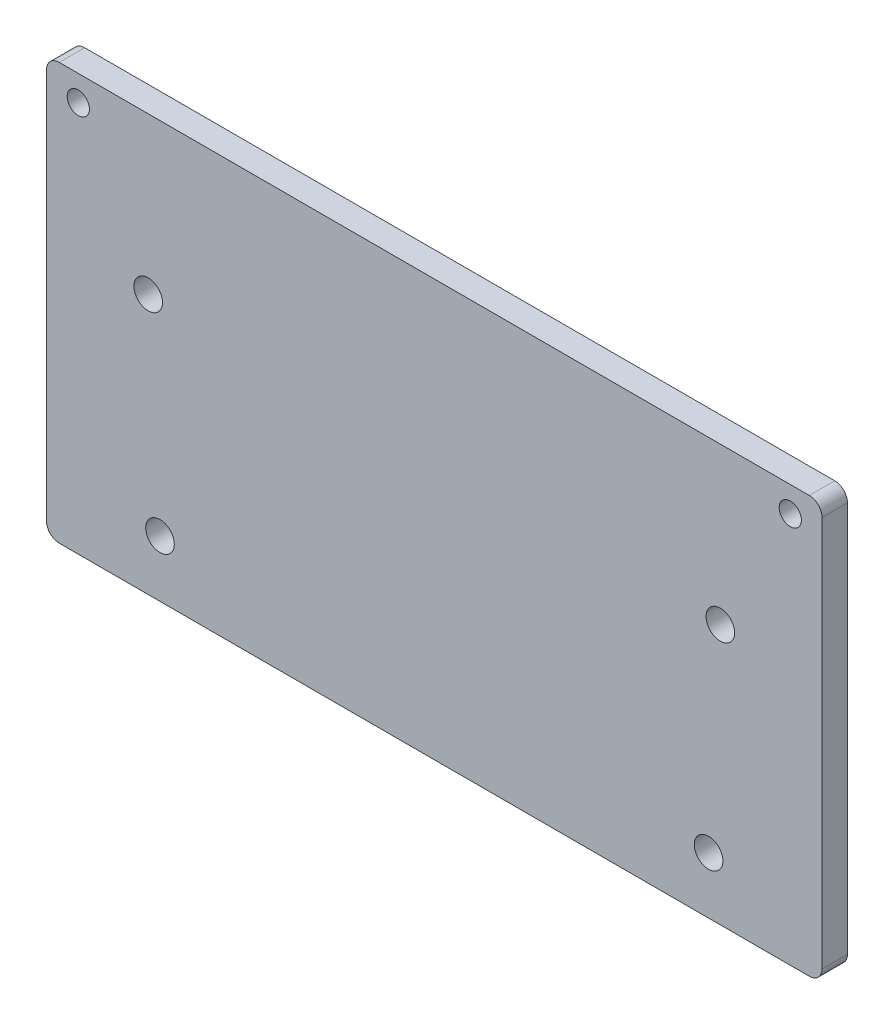
SolidWorks part; units mm, degrees
material "SUS201"
ref_plane "前视基准面" through (0, 0, 0) normal (0, 0, 1) x (1, 0, 0)
ref_plane "上视基准面" through (0, 0, 0) normal (0, 1, 0) x (1, 0, 0)
ref_plane "右视基准面" through (0, 0, 0) normal (1, 0, 0) x (0, 0, -1)
sketch "草图1" plane through (0, 0, 0) normal (0, 0, 1) x (1, 0, 0)
  line L0 (-45, 8.15) -> (45, 8.15) construction
  line L1 (-61, 32.75) -> (61, 32.75)
  line L2 (-61, 32.75) -> (-61, -32.75)
  line L3 (-61, -32.75) -> (61, -32.75)
  line L4 (61, 32.75) -> (61, -32.75)
  line L5 (-61, 32.75) -> (61, -32.75) construction
  line L6 (-61, -32.75) -> (61, 32.75) construction
  line L7 (0, 0) -> (0, 32.75) construction
  circle A0 centre (-56, 28.75) radius 1.75
  circle A1 centre (-45, 8.15) radius 2.25
  circle A2 centre (45, 8.15) radius 2.25
  circle A3 centre (56, 28.75) radius 1.75
  circle A4 centre (-43.15, -23.85) radius 2.25
  circle A5 centre (43.15, -23.85) radius 2.25
  point P0 (0, 0)
  dimension "D4" = 3.5
  dimension "D5" = 4.5
  dimension "D7" = 4
  dimension "D8" = 90
  dimension "D2" = 65.5
  dimension "D10" = 4.5
  dimension "D1" = 122
  dimension "D3" = 40.9
  dimension "D6" = 5
extrude "凸台-拉伸1" add sketch "草图1" along normal mid plane 4
fillet "圆角1" radius 2 4 edges at (61, -32.75, 0) (61, 32.75, 0) (-61, -32.75, 0) (-61, 32.75, 0)
